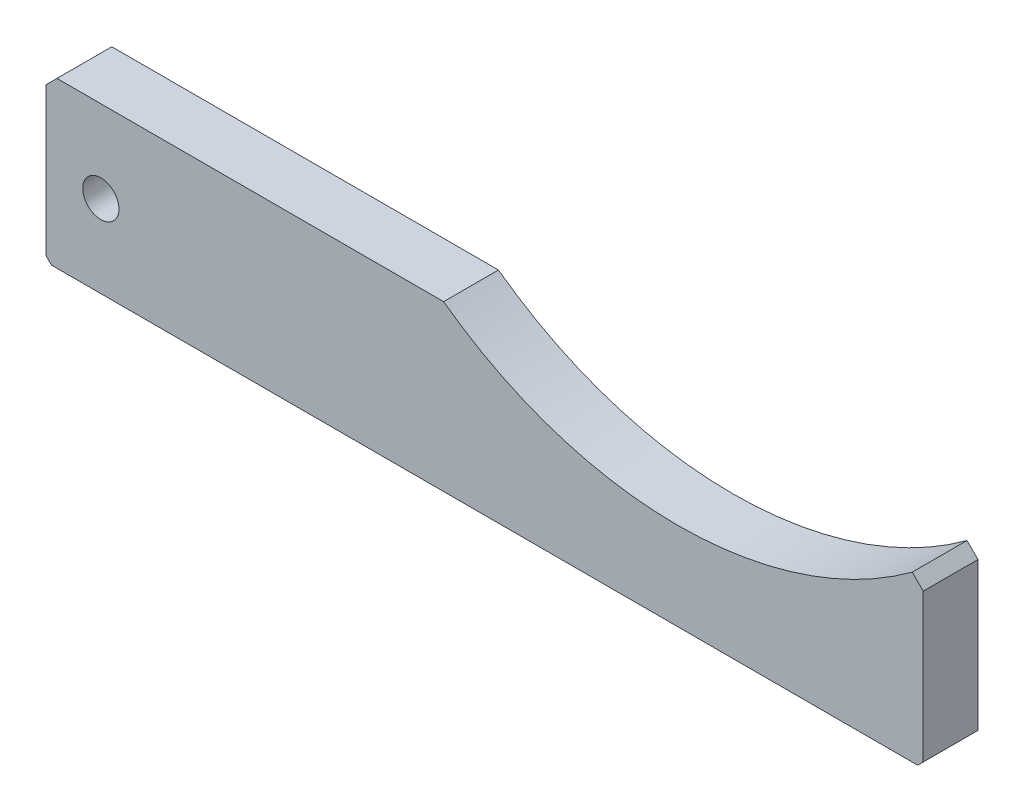
from build123d import *

# Parameters (mm, degrees)
SKETCH_1_W          = 160
SKETCH_1_H          = 30
EXTRUDE_1_DEPTH     = 10
CHAMFER_1_SIZE      = 2
CHAMFER_2_SIZE      = 1
HOLE_WIZARD_M6_1_D  = 6.6
CUT_EXTRUDE_1_DEPTH = 83.006097334


with BuildPart() as part:
    # 草图1 → 凸台-拉伸1 (new body)
    with BuildSketch(Plane.XY):
        Rectangle(SKETCH_1_W, SKETCH_1_H)
    extrude(amount=EXTRUDE_1_DEPTH)

    # 倒角1
    chamfer_1_edges = [part.edges().sort_by_distance(p)[0] for p in [
        (-80, 15, 5),
        (80, 15, 5),
    ]]
    chamfer(chamfer_1_edges, length=CHAMFER_1_SIZE)

    # 倒角2
    chamfer_2_edges = [part.edges().sort_by_distance(p)[0] for p in [
        (80, -15, 5),
        (-80, -15, 5),
    ]]
    chamfer(chamfer_2_edges, length=CHAMFER_2_SIZE)

    # M6 间隙孔1 (through all)
    with Locations(Plane.XY.offset(10)):
        with Locations((-70, 0)):
            Hole(HOLE_WIZARD_M6_1_D / 2)

    # 草图4 → 切除-拉伸1 (cut, through all)
    with BuildSketch(Plane.XY.offset(10)):
        with BuildLine():
            Line((-7.46846906, 15), (78, 15))
            ThreePointArc((78, 15), (35.26576547, 1.017096174), (-7.46846906, 15))
        make_face()
    extrude(amount=-CUT_EXTRUDE_1_DEPTH, mode=Mode.SUBTRACT)


solid = part.part
